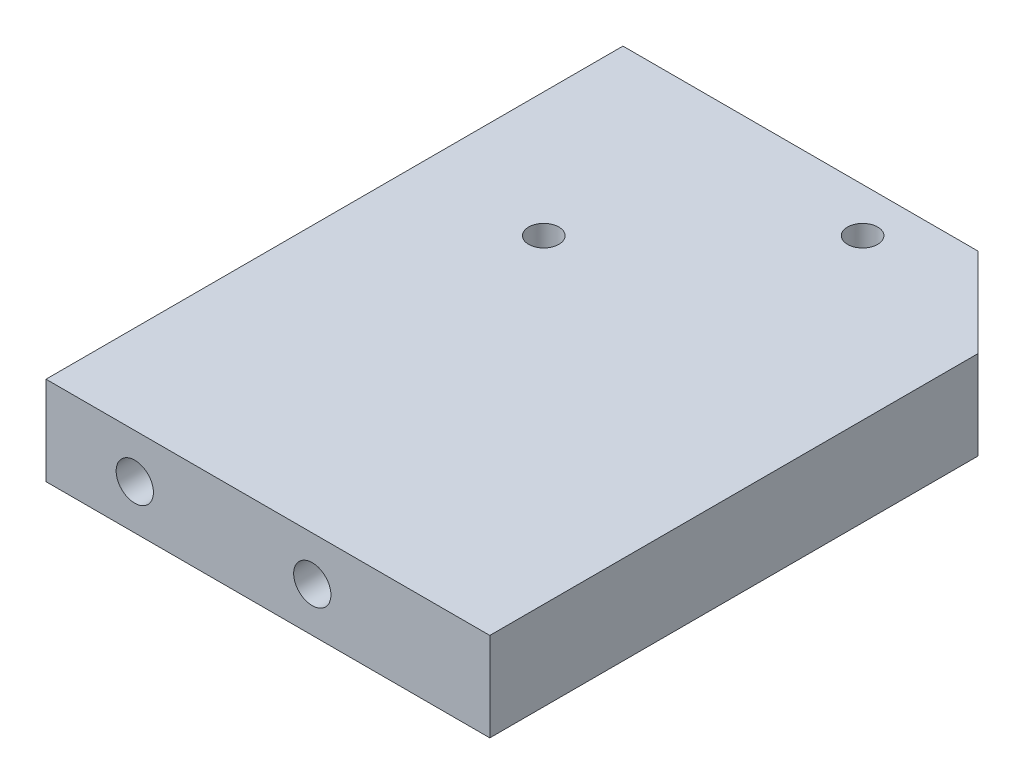
SolidWorks part; units mm, degrees
material "AL6061"
ref_plane "前视基准面" through (0, 0, 0) normal (0, 0, 1) x (1, 0, 0)
ref_plane "上视基准面" through (0, 0, 0) normal (0, 1, 0) x (1, 0, 0)
ref_plane "右视基准面" through (0, 0, 0) normal (1, 0, 0) x (0, 0, -1)
sketch "草图1" plane through (0, 0, 0) normal (0, 1, 0) x (1, 0, 0)
  line L1 (-25, 32.5) -> (25, 32.5)
  line L2 (-25, 32.5) -> (-25, -32.5)
  line L3 (-25, -32.5) -> (25, -32.5)
  line L4 (25, 32.5) -> (25, -32.5)
  line L5 (-25, 32.5) -> (25, -32.5) construction
  line L6 (-25, -32.5) -> (25, 32.5) construction
  point P0 (0, 0)
  dimension "D1" = 50
  dimension "D2" = 65
extrude "凸台-拉伸1" add sketch "草图1" along normal mid plane 10
chamfer "倒角1" distance 10 angle 45 1 edges at (25, 0, -32.5)
sketch "草图2" plane through (-25, 0, 0) normal (-1, 0, 0) x (0, 0, 1)
  line L0 (0, 0) -> (0, 10.9398) construction
  line L1 (-32.5, 5) -> (-32.5, -5) construction
  point P0 (-12.5, 0)
  point P10 (12.5, 0)
  dimension "D1" = 20
hole_wizard "M5 螺纹孔1" positions "草图2" profile "草图3" tap size "M5" standard "ISO"
sketch "草图3" plane through (-25, 0, -12.5) normal (0, 1, 0) x (0, 0, 1)
  line L0 (0, 0) -> (0, 13.6618)
  line L1 (0, 13.6618) -> (2.1, 12.4)
  line L2 (2.1, 12.4) -> (2.1, 0)
  line L5 (2.1, 0) -> (0, 0)
  line L10 (0, 13.6618) -> (-2.1, 12.4) construction
  line L11 (0, -6.35) -> (0, 107.95) construction
  dimension "螺纹孔钻头直径" = 4.2
  dimension "螺纹孔钻头深度" = 12.4
  dimension "导头角度" = 118
cosmetic thread "孔螺蚊线1" parameters "D1"=10, "D2"=5
cosmetic thread "孔螺蚊线2" parameters "D1"=10, "D2"=5
sketch "草图4" plane through (0, 0, 32.5) normal (0, 0, 1) x (1, 0, 0)
  line L2 (-25, 5) -> (-25, -5) construction
  line L3 (5, 0) -> (-15, 0) construction
  line L5 (-25, 5) -> (25, 5) construction
  point P0 (-15, 0)
  point P13 (5, 0)
  dimension "D1" = 10
  dimension "D2" = 20
  dimension "D3" = 5
sketch "草图6" plane through (0, -5, 0) normal (0, -1, 0) x (-1, 0, 0)
  point P0 (-7, 27.5)
  point P3 (10.9605, 9.5395)
hole_wizard "M3 六角凹头螺钉的柱形沉头孔1" positions "草图6" profile "草图7" counterbore size "M3" standard "ISO" end condition through all
sketch "草图7" plane through (7, -5, -27.5) normal (1, 0, 0) x (0, 0, -1)
  line L0 (0, 0) -> (0, 10)
  line L1 (0, 10) -> (1.7, 10)
  line L3 (1.7, 10) -> (1.7, 3.4)
  line L4 (1.7, 3.4) -> (3.25, 3.4)
  line L5 (3.25, 3.4) -> (3.25, 0)
  line L7 (3.25, 0) -> (0, 0)
  line L11 (0, -6.35) -> (0, 107.95) construction
  dimension "通孔孔直径" = 3.4
  dimension "通孔孔深度" = 10
  dimension "柱形沉头孔直径" = 6.5
  dimension "柱形沉头孔深度" = 3.4
hole_wizard "M5 螺纹孔2" positions "草图4" profile "草图5" tap size "M5" standard "ISO"
sketch "草图5" plane through (-15, 0, 32.5) normal (1, 0, 0) x (0, -1, 0)
  line L0 (0, 0) -> (0, 13.6618)
  line L1 (0, 13.6618) -> (2.1, 12.4)
  line L2 (2.1, 12.4) -> (2.1, 0)
  line L5 (2.1, 0) -> (0, 0)
  line L10 (0, 13.6618) -> (-2.1, 12.4) construction
  line L11 (0, -6.35) -> (0, 107.95) construction
  dimension "螺纹孔钻头直径" = 4.2
  dimension "螺纹孔钻头深度" = 12.4
  dimension "导头角度" = 118
cosmetic thread "孔螺蚊线3" parameters "D1"=10, "D2"=5
cosmetic thread "孔螺蚊线4" parameters "D1"=10, "D2"=5
sketch "草图8" plane through (0, -5, 0) normal (0, 1, 0) x (1, 0, 0)
  line L0 (25, -32.5) -> (25, 22.5) construction
  line L1 (-25, -32.5) -> (25, -32.5)
  line L2 (-25, -32.5) -> (-25, -17.5)
  line L3 (-25, -17.5) -> (25, -17.5)
  line L4 (25, -32.5) -> (25, -17.5)
  dimension "D1" = 15
extrude "凸台-拉伸2" [suppressed] add sketch "草图8" against normal blind 5
chamfer "倒角2" [suppressed] distance 5 angle 45
